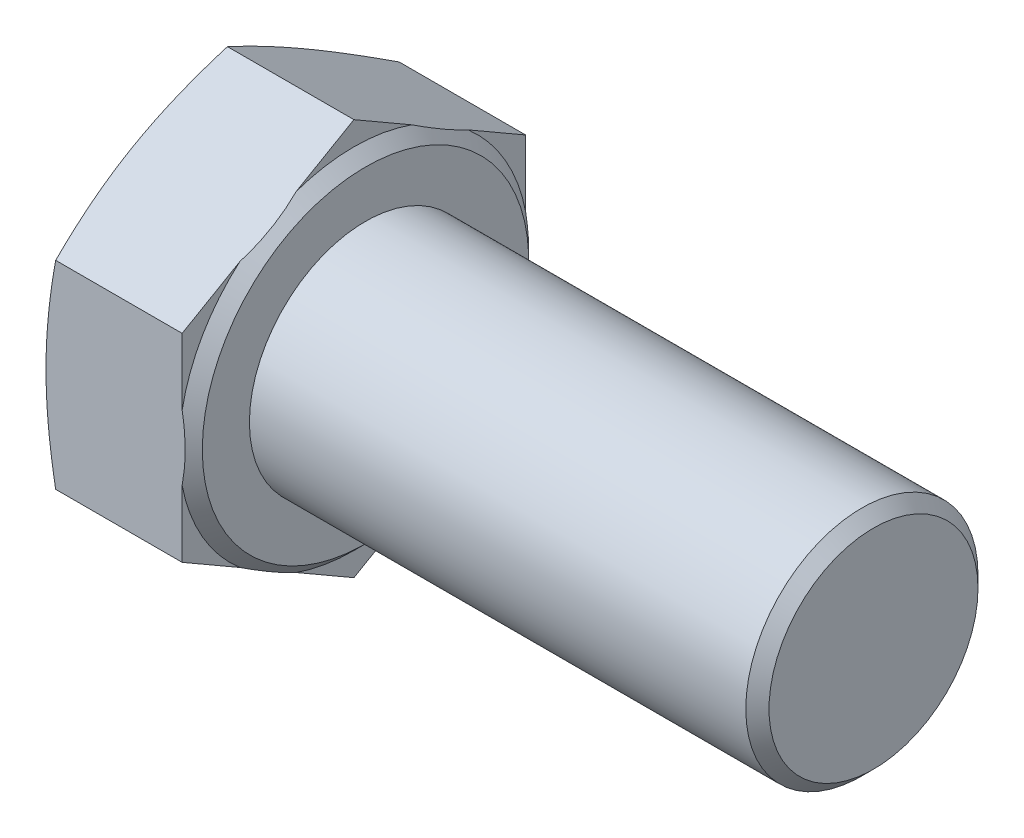
SolidWorks part; units mm, degrees
ref_plane "Front" through (0, 0, 0) normal (0, 0, 1) x (1, 0, 0)
ref_plane "Top" through (0, 0, 0) normal (0, 1, 0) x (1, 0, 0)
ref_plane "Right" through (0, 0, 0) normal (1, 0, 0) x (0, 0, -1)
other "Configuration Table"
sketch "Sketch2" plane through (0, 0, 0) normal (1, 0, 0) x (0, 0, -1)
  line L1 (11.835, -6.8329) -> (11.835, 6.8329)
  line L2 (11.835, 6.8329) -> (0, 13.6659)
  line L3 (0, 13.6659) -> (-11.835, 6.8329)
  line L4 (-11.835, 6.8329) -> (-11.835, -6.8329)
  line L5 (-11.835, -6.8329) -> (0, -13.6659)
  line L6 (0, -13.6659) -> (11.835, -6.8329)
  circle A0 centre (0, 0) radius 11.835 construction
extrude "BaseHead" add sketch "Sketch2" along normal blind 10.18
sketch "Sketch3" plane through (0, 0, 0) normal (0, 0, 1) x (1, 0, 0)
  line L0 (10.18, 13.6659) -> (10.18, 11.245)
  line L2 (10.18, 11.245) -> (9.38, 12.045)
  line L3 (9.38, 12.045) -> (9.38, 13.6659)
  line L5 (9.38, 13.6659) -> (10.18, 13.6659)
  line L6 (-0.9571, 0) -> (7.6478, 0) construction
  line L7 (10.18, 13.6659) -> (0, 13.6659) construction
  dimension "D1" = 45
  dimension "c" = 0.8
  dimension "Dw" = 22.49
revolve "BearingFace" cut sketch "Sketch3" angle 360 about L6
sketch "Sketch4" plane through (0, 0, 0) normal (0, 0, 1) x (1, 0, 0)
  line L0 (-0.4935, 0) -> (3.5626, 0) construction
  line L2 (0, 13.6659) -> (0.6664, 13.6659)
  line L4 (0.6664, 13.6659) -> (0, 11.835)
  line L6 (0, 11.835) -> (0, 13.6659)
  line L7 (9.38, 13.6659) -> (0, 13.6659) construction
revolve "HeadChamfer" cut sketch "Sketch4" angle 360 about L0
sketch "Sketch5" plane through (10.18, 0, 0) normal (1, 0, 0) x (0, 0, -1)
  circle A0 centre (0, 0) radius 8
extrude "BaseBody" add sketch "Sketch5" along normal blind 35
cosmetic thread "ThreadCosmetic1" [suppressed] parameters "D2"=13.835
chamfer "Chamfer1" distance 0.8 angle 45 1 edges at (45.18, 0, -8)
fillet "HeadFillet" [suppressed] radius 0.6
sketch "Sketch6" plane through (0, 0, 0) normal (0, 0, 1) x (1, 0, 0)
  line L0 (10.18, 9.0825) -> (11.2625, 9.0825)
  line L1 (11.2625, 9.0825) -> (11.2625, 8)
  line L2 (11.2625, 8) -> (10.7213, 7.0625)
  line L3 (10.7213, 7.0625) -> (10.18, 8)
  line L4 (10.18, 8) -> (10.18, 9.0825)
  line L5 (44.38, 8) -> (10.18, 8) construction
  line L6 (10.18, -11.245) -> (10.18, 11.245) construction
revolve "Cut-Revolve10" [suppressed] cut sketch "Sketch6" angle 360 about axis through (-0.9571, 0, 0) along (1, 0, 0)
pattern_linear "LPattern10" [suppressed] count 27
equation "\"D2@Sketch4\" = \"s@Sketch2\""
equation "\"D1@Chamfer1\" = 0.05 * \"d@Sketch5\""
equation "\"D1@Sketch6\" =  ( \"d@Sketch5\" - \"D2@ThreadCosmetic1\" )  / 2"
equation "\"pitch@LPattern10\" = \"D1@Sketch6\" * 1.2"
equation "\"D1@LPattern10\" = \"l@BaseBody\" / \"pitch@LPattern10\""
